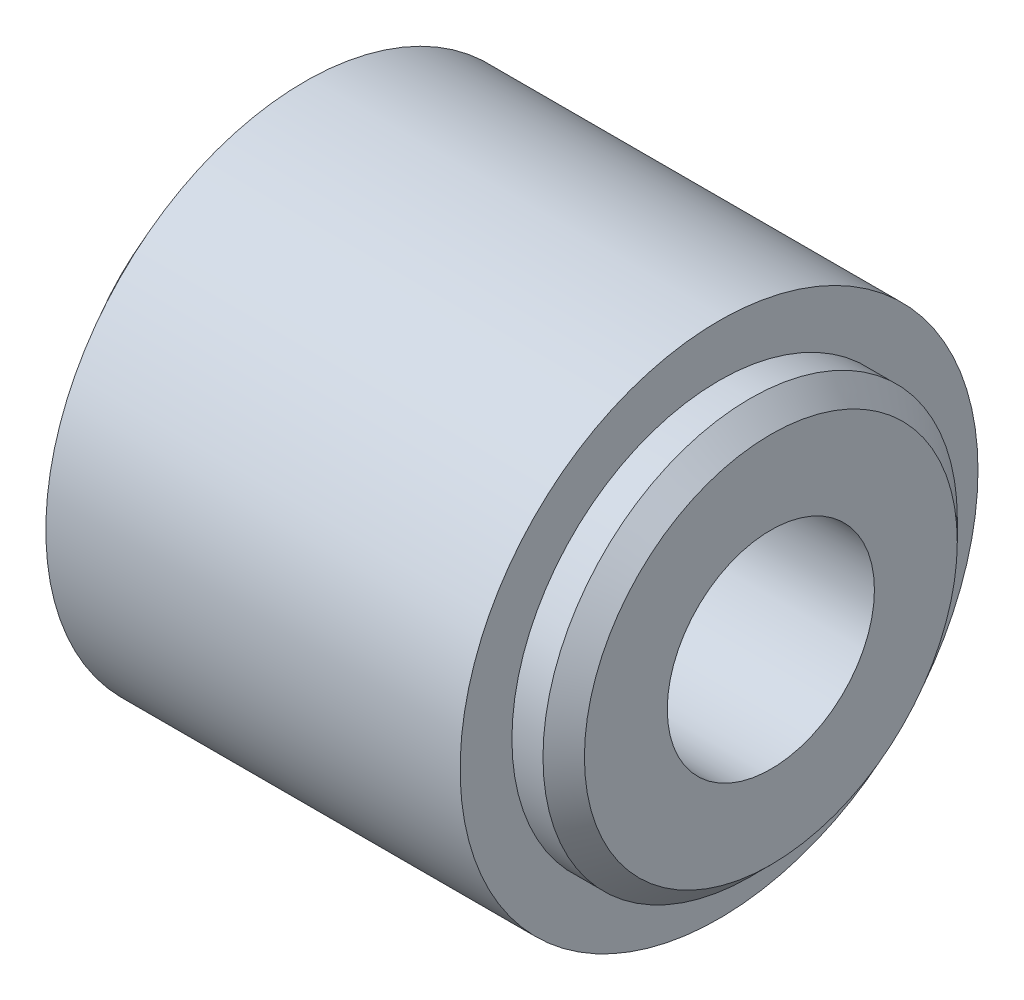
SolidWorks part; units mm, degrees
ref_plane "前视基准面" through (0, 0, 0) normal (0, 0, 1) x (1, 0, 0)
ref_plane "上视基准面" through (0, 0, 0) normal (0, 1, 0) x (1, 0, 0)
ref_plane "右视基准面" through (0, 0, 0) normal (1, 0, 0) x (0, 0, -1)
sketch "草图1" plane through (0, 0, 0) normal (1, 0, 0) x (0, 0, -1)
  circle A0 centre (0, 0) radius 5
  circle A1 centre (0, 0) radius 10
extrude "凸台-拉伸1" add sketch "草图1" along normal mid plane 25
sketch "草图2" plane through (0, 0, 0) normal (1, 0, 0) x (0, 0, -1)
  circle A0 centre (0, 0) radius 12.5
  circle A1 centre (0, 0) radius 10
extrude "凸台-拉伸2" add sketch "草图2" along normal mid plane 20
chamfer "倒角1" distance 1 angle 45 2 edges at (-12.5, 0, -10) (12.5, 0, -10)
